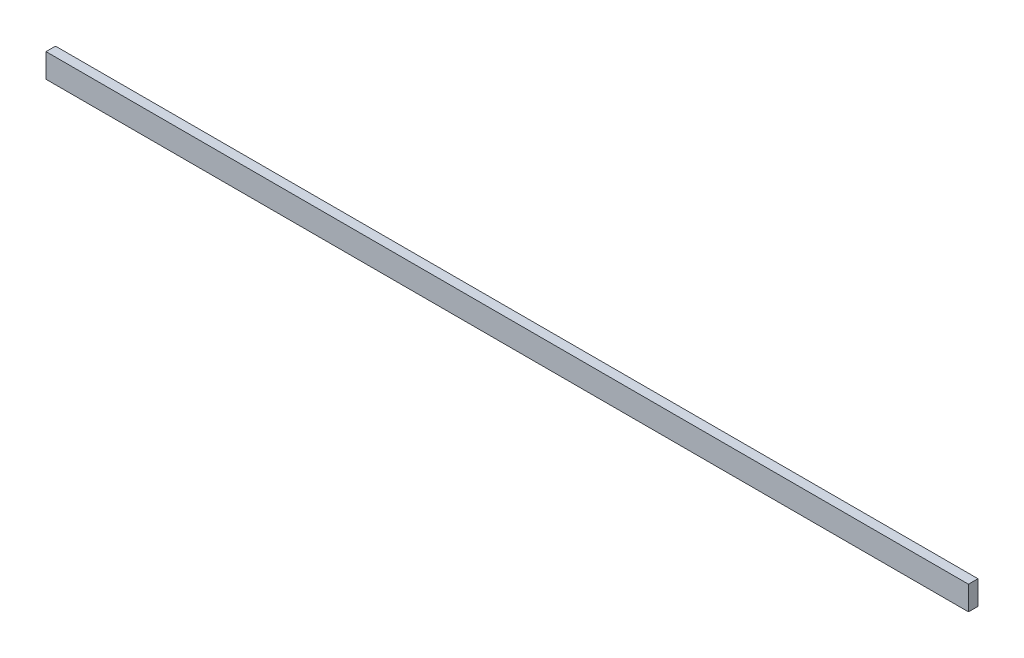
from build123d import *

# Parameters (mm, degrees)
SKETCH1_W           = 2425
SKETCH1_H           = 63
BOSS_EXTRUDE1_DEPTH = 25


with BuildPart() as part:
    # Sketch1 → Boss-Extrude1 (new body)
    with BuildSketch(Plane.XY):
        with Locations((1212.5, 31.5)):
            Rectangle(SKETCH1_W, SKETCH1_H)
    extrude(amount=BOSS_EXTRUDE1_DEPTH)


solid = part.part
